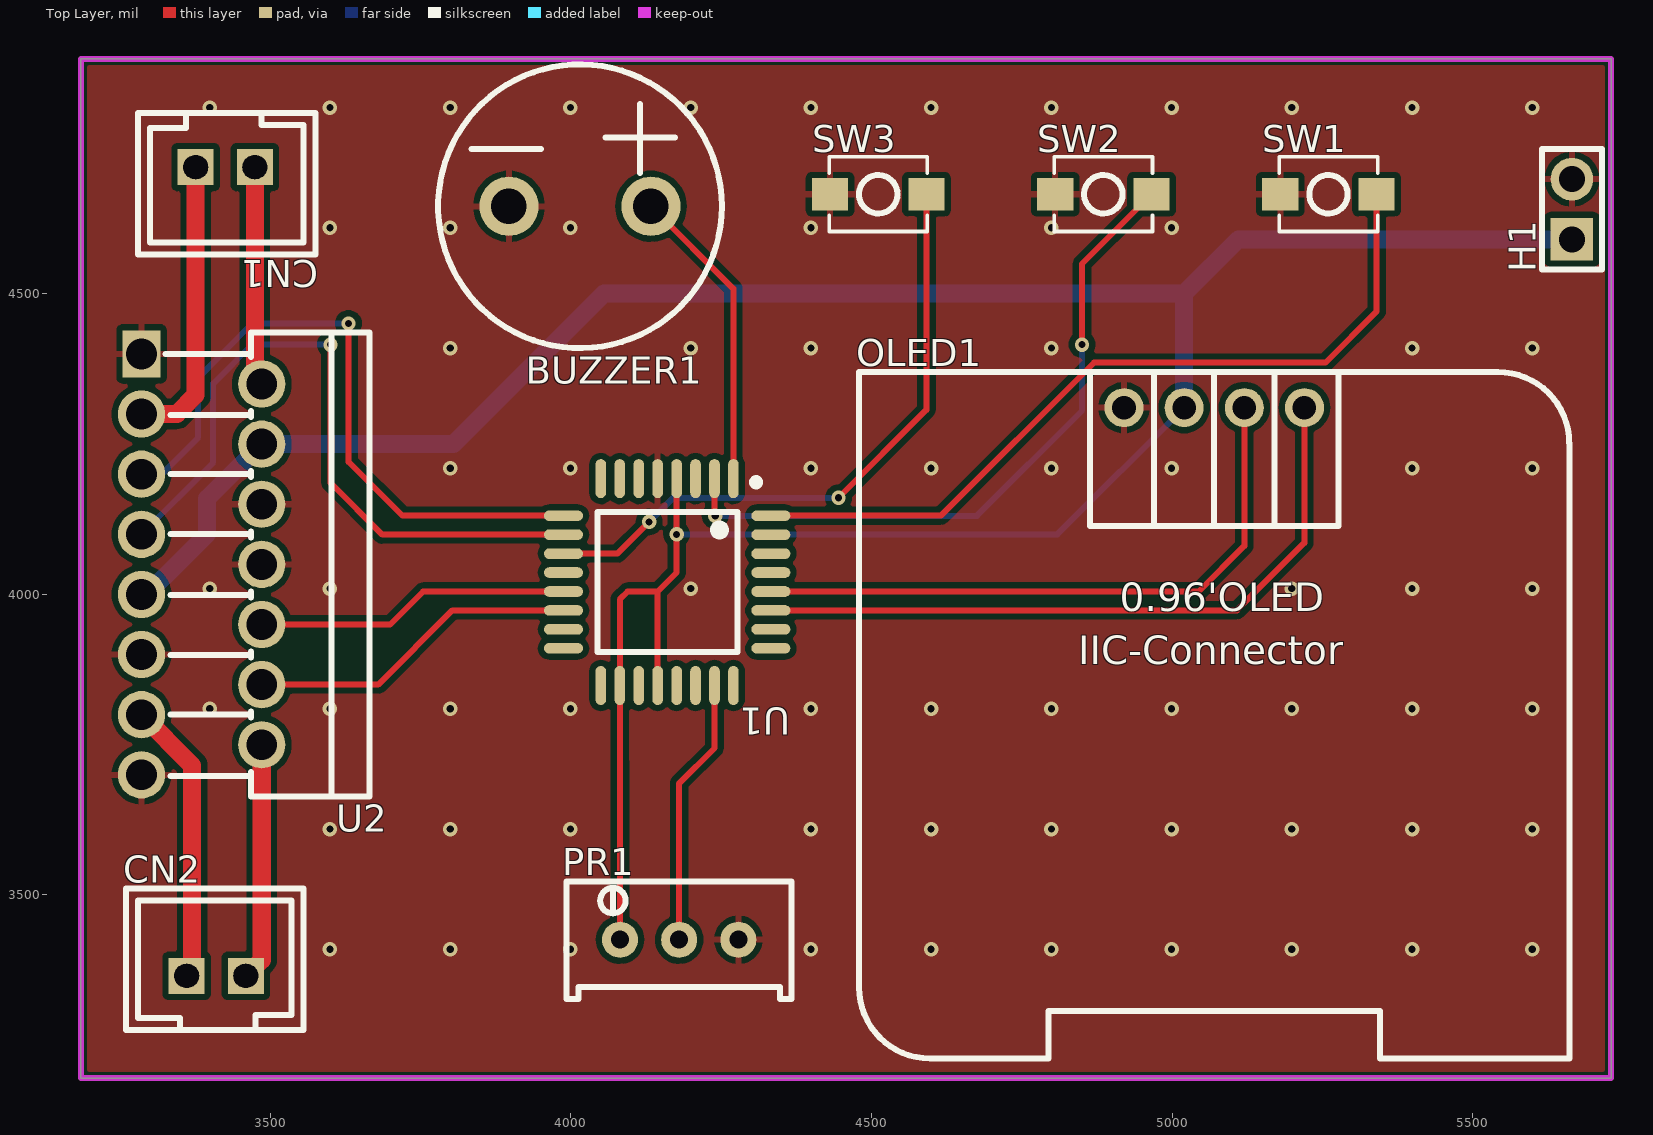
[diagram p0: Top Layer view]
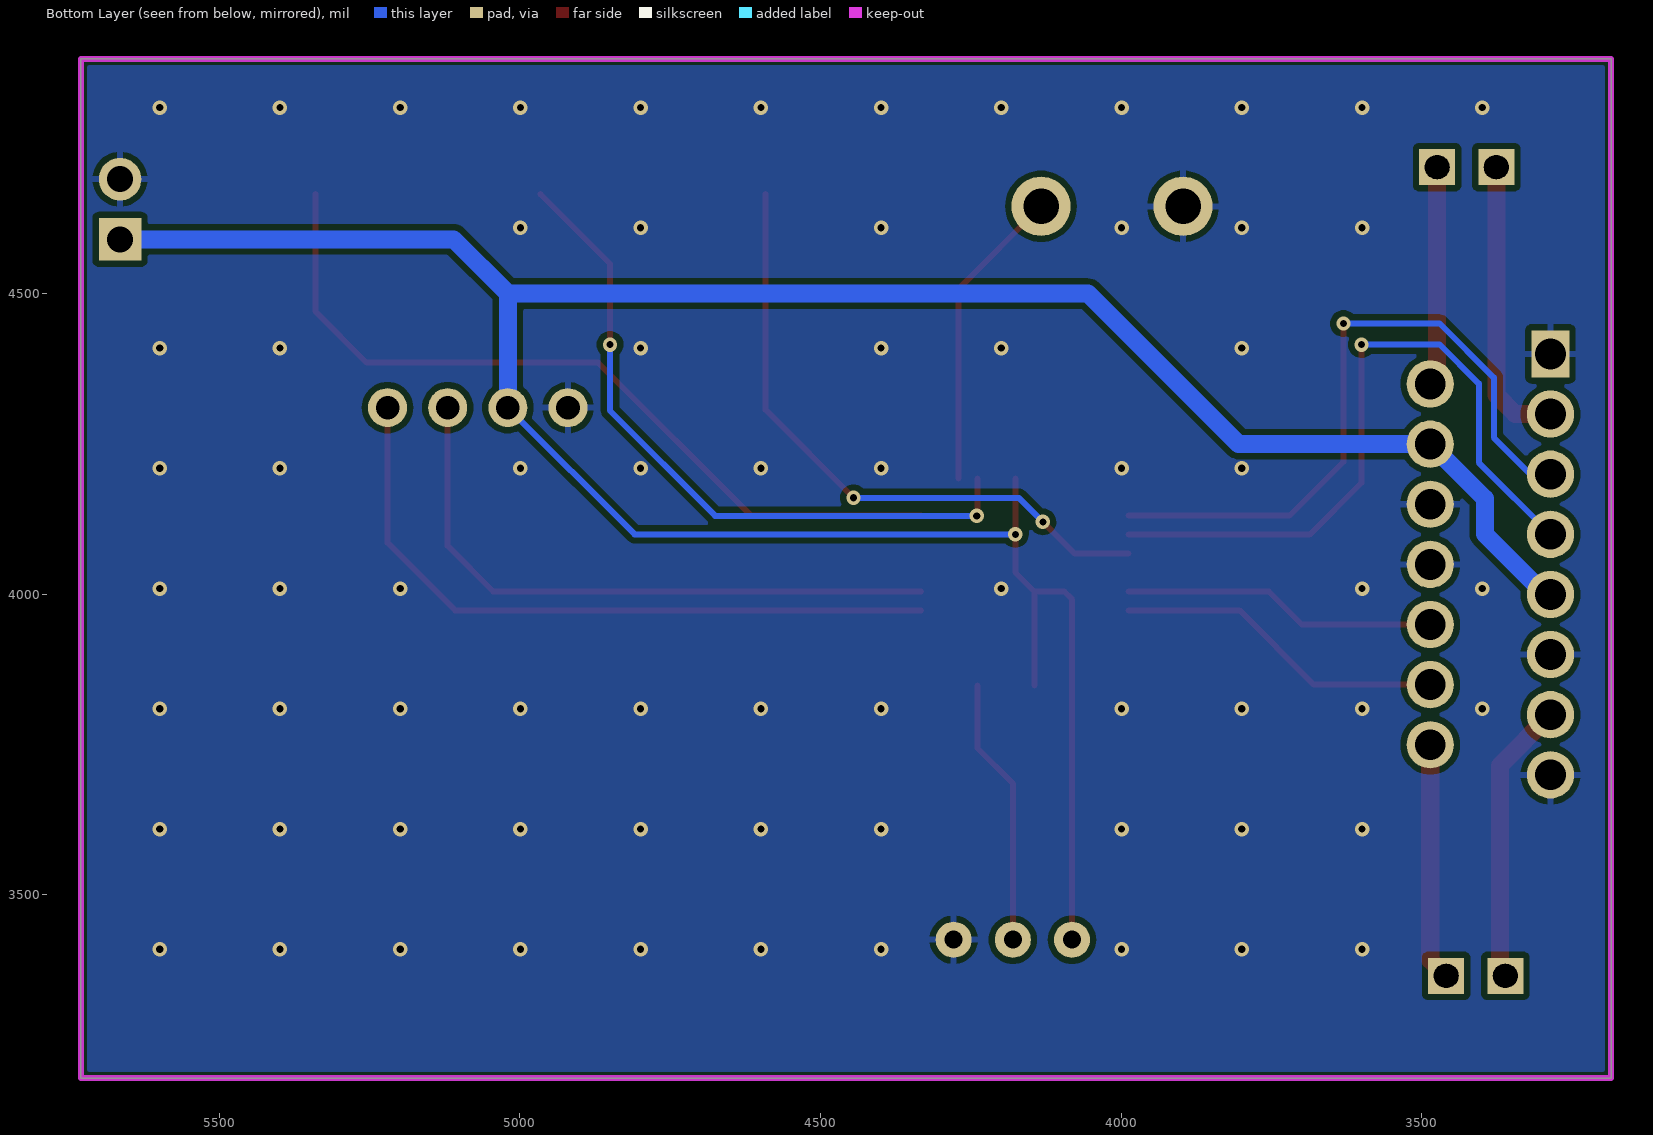
[diagram p1: Bottom Layer view, seen from below]
# Altium PCB MISC52152.pcbdoc
Units mil, origin at the board's own origin, x right, y up, seen from the top; angles counter-clockwise.
Board outline 2545 x 1695 mil, 2 copper layers (Top Layer, Bottom Layer), stack 62.206 mil thick; 11 components, 17 nets, 68 pads, 76 vias.

## Layer stack, top to bottom
Top Solder Mask Layer: solder mask 0.394, Dk 3.3
Top Layer: signal copper 1.379
Dielectric1: surface 59.449, FR4, Dk 4.5
Bottom Layer: signal copper 1.378
Bottom Solder Mask Layer: solder mask 0.394, Dk 3.3

## Board outline
3185,4890 3185,3195 5730,3195 5730,4890

## Design rules (kind name [scope] priority, off if disabled: settings)
BoardOutlineClearance copperThickness2oz_1 [All] p2 off: genericclearance=7.99 ignorepadtopadclearanceinfootprint=FALSE except(0: Arc-SplitContinuation Track-SplitContinuation SMDPad-SplitContinuation THPad-SplitContinuation Via-SplitContinuation Fill-SplitContinuation Region-SplitContinuation Poly-SplitContinuation Text-SplitContinuation Hole-SplitContinuation; 5.98: Arc-CutoutEdge SMDPad-CutoutEdge THPad-CutoutEdge Via-CutoutEdge Fill-CutoutEdge Region-CutoutEdge Text-CutoutEdge; 6.93: Hole-OutlineEdge Hole-CutoutEdge; 10: Poly-OutlineEdge Poly-CutoutEdge; 11.81: Arc-OutlineEdge Track-OutlineEdge SMDPad-OutlineEdge THPad-OutlineEdge Via-OutlineEdge Fill-OutlineEdge Region-OutlineEdge Text-OutlineEdge Track-CutoutEdge)
BoardOutlineClearance copperThickness1oz_1 [All] p4: genericclearance=4.02 ignorepadtopadclearanceinfootprint=FALSE except(0: Arc-SplitContinuation Track-SplitContinuation SMDPad-SplitContinuation THPad-SplitContinuation Via-SplitContinuation Fill-SplitContinuation Region-SplitContinuation Poly-SplitContinuation Text-SplitContinuation Hole-SplitContinuation; 6: SMDPad-CutoutEdge THPad-CutoutEdge Via-CutoutEdge Fill-CutoutEdge Region-CutoutEdge Text-CutoutEdge; 6.93: Hole-OutlineEdge Hole-CutoutEdge; 10: Poly-OutlineEdge Poly-CutoutEdge; 11.8: Arc-OutlineEdge Track-OutlineEdge SMDPad-OutlineEdge THPad-OutlineEdge Via-OutlineEdge Fill-OutlineEdge Region-OutlineEdge Text-OutlineEdge; 11.81: Arc-CutoutEdge Track-CutoutEdge)
Clearance copperThickness2oz [All] p1 off: gap=7.99 ignorepadtopadclearanceinfootprint=FALSE except(5.98: SMDPad-Track SMDPad-SMDPad THPad-Track SMDPad-THPad THPad-THPad Track-Via SMDPad-Via THPad-Via Via-Via Fill-Track Region-Track Fill-SMDPad Region-SMDPad Fill-THPad Region-THPad Fill-Via Region-Via Fill-Fill Fill-Region Region-Region Arc-Track Arc-SMDPad Arc-THPad Arc-Via Fill-Arc Region-Arc Arc-Arc Text-Track SMDPad-Text Text-THPad Text-Via Fill-Text Region-Text Arc-Text Text-Text; 6.93: Hole-Track Hole-SMDPad Hole-THPad Hole-Via Fill-Hole Region-Hole Hole-Arc Hole-Text; 10: Poly-Track Poly-SMDPad Poly-THPad Poly-Via Poly-Fill Poly-Region Poly-Poly Poly-Arc Poly-Text Poly-Hole)
Clearance copperThickness1oz [All] p3: gap=4.02 ignorepadtopadclearanceinfootprint=FALSE except(5.98: SMDPad-Track SMDPad-SMDPad THPad-Track SMDPad-THPad THPad-THPad Track-Via SMDPad-Via THPad-Via Via-Via Fill-Track Region-Track Fill-SMDPad Region-SMDPad Fill-THPad Region-THPad Fill-Via Region-Via Fill-Fill Fill-Region Region-Region; 6: Arc-Track Arc-SMDPad Arc-THPad Arc-Via Fill-Arc Region-Arc Arc-Arc Text-Track SMDPad-Text Text-THPad Text-Via Fill-Text Region-Text Arc-Text Text-Text; 6.93: Hole-Track Hole-SMDPad Hole-THPad Hole-Via Fill-Hole Region-Hole Hole-Arc Hole-Text; 10: Poly-Track Poly-SMDPad Poly-THPad Poly-Via Poly-Fill Poly-Region Poly-Poly Poly-Arc Poly-Text Poly-Hole)
DiffPairsRouting differentialPair [All] p1: maxlimit=6 minlimit=6 mostfreqgap=6 toplayer_minwidth=5 toplayer_prefwidth=10 toplayer_maxwidth=100 toplayer_mingap=6 toplayer_prefgap=6 toplayer_maxgap=6 bottomlayer_minwidth=5 bottomlayer_prefwidth=10 bottomlayer_maxwidth=100 bottomlayer_mingap=6 bottomlayer_prefgap=6 bottomlayer_maxgap=6 maxuncoupledlength=10
HoleToHoleClearance otherClearance [All] p1: gap=11.81 allowstackedmicrovias=TRUE
Length netLength [All] p1: minlimit=0 maxlimit=0
MatchedLengths netLengthTolerance [All] p1: tolerance=1000
PasteMaskExpansion pasteMaskExpansion [All] p1: expansion=0
PlaneConnect innerPlane [All] p1: planeconnectstyle=Relief reliefexpansion=20 reliefentries=4 reliefconductorwidth=10 reliefairgap=10
PolygonConnect copperRegion [(InNet('GND'))] p1: connectstyle=Relief reliefconductorwidth=10 reliefentries=4 polygonreliefangle="90 Angle" airgapwidth=10 via.connectstyle=Relief via.reliefconductorwidth=10 via.reliefentries=4 via.polygonreliefangle="90 Angle" via.airgapwidth=10
RoutingVias viaSize [All] p1: holewidth=12.01 width=24.02 viastyle="Through Hole" minholewidth=11.81 minwidth=19.68 maxholewidth=248.03 maxwidth=393.7
SolderMaskExpansion solderMaskExpansion [IsVia] p1: expansion=-1000 istentingtop=TRUE
SolderMaskExpansion solderMaskExpansion [All] p2: expansion=2 istentingtop=FALSE
Width copperThickness2oz_2 [All] p1 off: maxlimit=100 minlimit=8 preferedwidth=10
Width copperThickness1oz_2 [All] p2: maxlimit=100 minlimit=5 preferedwidth=10

## Components (designator, comment, footprint, x,y, rotation, side; value= is the part's Value field where it differs from the comment)
BUZZER1 "buzzer" BUZ-TH_BD12.0-P6.00-D0.9-RD 4015,4645 r0 top
CN1 "XH2.54-2PIN-直针" CONN-TH_XH2.54-2P 3424.99,4709.99 r180 top
CN2 "XH2.54-2PIN-直针" CONN-TH_XH2.54-2P 3410,3365 r0 top
H1 "" HDR-TH_2P-P2.54-V-M-1 5665,4640 r90 top
OLED1 "" 0.96OLED_4P 5070,4310 r0 top
PR1 "10kΩ" R_3296 4180,3430 r0 top
SW1 "" Key_SMD_3x4x2 5260,4665 r0 top
SW2 "" Key_SMD_3x4x2 4885.6,4665 r0 top
SW3 "" Key_SMD_3x4x2 4511.19,4665 r0 top
U1 "ATMEGA328PB-AUR" TQFP-32_L7.0-W7.0-P0.80-LS9.0-BL 4160,4020 r180 top
U2 "L298N" MULTIWATT-15_L19.6-W5.0-P1.27-L 3385.7,4049.36 r270 top

## Footprints (in the part's own frame and the unit in brackets; to place one, negate y for a bottom-side part, rotate by r counter-clockwise, add the part's x,y. Pads: shape width x height; smd on the part's side, far side on the other; paste and mask are expansions set on the pad)
0.96OLED_4P [mm]
  round 1.65 hole 1 copper offset 0,0: 1(-3.81,-0.001) 2(-1.27,0.002) 3(1.27,0.002) 4(3.81,0.002)
  silkscreen extent -15,-27.5 15,1.5
BUZ-TH_BD12.0-P6.00-D0.9-RD [mm]
  round 2.5 hole 1.5 paste+0 mask+0.05: 1(-3,0) 2(3,0)
  silkscreen extent -5.99,-5.99 5.99,5.99
CONN-TH_XH2.54-2P [mil]
  rect 60x60 hole 39.37 slot 41.34 at 0 deg paste+0 mask+1.97: 1(-49.22,0) 2(49.21,0)
  silkscreen extent -150,-90 145,145
HDR-TH_2P-P2.54-V-M-1 [mm]
  rect 1.8x1.8 hole 1.1: 1(-1.27,0)
  round 1.8 hole 1.1: 2(1.27,0)
  silkscreen extent -2.54,-1.27 2.54,1.27
Key_SMD_3x4x2 [mm]
  rect 1.53x1.36 smd paste+0 mask+0.051: 1(-2.035,0) 2(2.035,0)
  silkscreen extent -2.08,-1.58 2.08,1.58
MULTIWATT-15_L19.6-W5.0-P1.27-L [mm]
  rect 2x1.6 hole 1.3: 1(-8.89,-2.54)
  round 2 hole 1.3: 2(-7.62,2.54) 3(-6.35,-2.54) 4(-5.08,2.54) 5(-3.81,-2.54) 6(-2.54,2.54) 7(-1.27,-2.54) 8(0,2.54) 9(1.27,-2.54) 10(2.54,2.54) 11(3.81,-2.54) 12(5.08,2.54) 13(6.35,-2.54) 14(7.62,2.54) 15(8.89,-2.54)
  silkscreen extent -9.8,-1.52 9.8,7.09
R_3296 [mil]
  round 60 hole 30 paste+0 mask+2: 1(-98.4,-5) 2(0,-5) 3(98.4,-5)
  silkscreen extent -187,-103 187,92
TQFP-32_L7.0-W7.0-P0.80-LS9.0-BL [mm]
  oval 0.45x1.65 smd: 1(-2.8,-4.369) 2(-2,-4.369) 3(-1.2,-4.369) 4(-0.4,-4.369) 5(0.4,-4.369) 6(1.2,-4.369) 7(2,-4.369) 8(2.8,-4.369) 17(2.8,4.369) 18(2,4.369) 19(1.2,4.369) 20(0.4,4.369) 21(-0.4,4.369) 22(-1.2,4.369) 23(-2,4.369) 24(-2.8,4.369)
  oval 1.65x0.45 smd: 9(4.381,-2.8) 10(4.381,-2) 11(4.381,-1.2) 12(4.381,-0.4) 13(4.381,0.4) 14(4.381,1.2) 15(4.381,2) 16(4.381,2.8) 25(-4.381,2.8) 26(-4.381,2) 27(-4.381,1.2) 28(-4.381,0.4) 29(-4.381,-0.4) 30(-4.381,-1.2) 31(-4.381,-2) 32(-4.381,-2.8)
  silkscreen extent -3.91,-4.36 2.94,2.95

## Via types
v1: diameter 24.02, hole 12, Top Layer to Bottom Layer, 76 vias

## Nets (pads, with @x,y where several pads share a name; then routed paths per layer and width w, separated by ;. In a path a pad name is that pad's centre, name@x,y a point inside that pad or via, vN(x,y) a via of type N, cw(c..) or ccw(c..) an arc to the next point about the centre after c; other vN are vias at no path point)
$1N37: CN1.1 U2.2 | length 365.4
  Top Layer w30: CN1.1 3474.21,4360.85 U2.2
$1N38: CN1.2 U2.3 | length 482.3
  Top Layer w30: U2.3 3344.36,4299.36 3375.78,4330.78 CN1.2
$1N39: CN2.1 U2.13 | length 473.1
  Top Layer w30: U2.13 3370,3715.06 3370,3374.22 CN2.1
$1N40: CN2.2 U2.14 | length 395.3
  Top Layer w30: CN2.2 3485.7,3391.48 U2.14
+5V: H1.1 OLED1.2 PR1.1 U1.4 U1.18 U1.20 U2.4 U2.9 | length 4771.7
  Top Layer w10: PR1.1 4081.6,3720.92 4081.26,3721.26 U1.18 4081.26,3991.26 4094.25,4004.25 4144.25,4004.25 ; U1.20 4144.25,4004.25 ; U1.4 v1(4175.75,4099.25) 4175.75,4035.75 4144.25,4004.25
  Bottom Layer w10: v1(4175.75,4099.25) 4809.2,4099.25 OLED1.2@5020,4310.05
  Bottom Layer w30: U2.9 3294.36,3999.36 3395,4100 3395,4158.67 U2.4 3804.36,4249.36 4055,4500 5020,4500 ; OLED1.2@5020,4310.05 5020,4500 ; H1.1 5110,4590 5020,4500
BTN_MODE: SW2.2 U1.2 | length 1152.9
  Top Layer w10: U1.2 4238.74,4131.26 v1(4240,4130) ; v1(4850,4415) 4850,4549.28 SW2.2
  Bottom Layer w10: v1(4240,4130) 4675,4130 4850,4305 v1(4850,4415)
BTN_START: SW1.2 U1.32 | length 1343.3
  Top Layer w10: U1.32 4615.24,4130.24 4870,4385 5255,4385 5340.12,4470.12 SW1.2
BTN_STOP: SW3.2 U1.11 | length 1061.5
  Top Layer w10: U1.11 4077.24,4067.24 v1(4130,4120) ; v1(4445,4160) 4591.31,4306.31 SW3.2
  Bottom Layer w10: v1(4130,4120) 4170,4160 v1(4445,4160)
BUZZER: BUZZER1.2 U1.1 | length 509.8
  Top Layer w10: BUZZER1.2 4270.24,4507.87 U1.1
GND: BUZZER1.1 H1.2 OLED1.1 PR1.3 SW1.1 SW2.1 SW3.1 U1.5 U2.1 U2.6 U2.8 U2.11 U2.15
  other v1: 3599.1,3409.1 3799.1,3409.1 3999.1,3409.1 4399.1,3409.1 4599.1,3409.1 4799.1,3409.1 4999.1,3409.1 5199.1,3409.1 5399.1,3409.1 5599.1,3409.1 3599.1,3609.1 3799.1,3609.1 3999.1,3609.1 4399.1,3609.1 4599.1,3609.1 4799.1,3609.1 4999.1,3609.1 5199.1,3609.1 5399.1,3609.1 5599.1,3609.1 3399.1,3809.1 3599.1,3809.1 3799.1,3809.1 3999.1,3809.1 4399.1,3809.1 4599.1,3809.1 4799.1,3809.1 4999.1,3809.1 5199.1,3809.1 5399.1,3809.1 5599.1,3809.1 3399.1,4009.1 3599.1,4009.1 4199.1,4009.1 5199.1,4009.1 5399.1,4009.1 5599.1,4009.1 3799.1,4209.1 3999.1,4209.1 4399.1,4209.1 4599.1,4209.1 4799.1,4209.1 4999.1,4209.1 5399.1,4209.1 5599.1,4209.1 3799.1,4409.1 4199.1,4409.1 4399.1,4409.1 4799.1,4409.1 5399.1,4409.1 5599.1,4409.1 3599.1,4609.1 3799.1,4609.1 3999.1,4609.1 4399.1,4609.1 4799.1,4609.1 4999.1,4609.1 3399.1,4809.1 3599.1,4809.1 3799.1,4809.1 3999.1,4809.1 4199.1,4809.1 4399.1,4809.1 4599.1,4809.1 4799.1,4809.1 4999.1,4809.1 5199.1,4809.1 5399.1,4809.1 5599.1,4809.1
IN1: U1.9 U2.5 | length 1131.4
  Top Layer w10: v1(3630,4450) 3630,4220 3719.76,4130.24 U1.9
  Bottom Layer w10: U2.5 3319.36,4199.36 3380,4260 3380,4360 3470,4450 v1(3630,4450)
IN2: U1.10 U2.7 | length 1175.2
  Top Layer w10: v1(3600,4415) 3600,4185 3686.26,4098.74 U1.10
  Bottom Layer w10: U2.7 3405,4218.67 3405,4350 3470,4415 v1(3600,4415)
IN3: U1.13 U2.10 | length 524.5
  Top Layer w10: U2.10 3699.36,3949.36 3754.25,4004.25 U1.13
IN4: U1.14 U2.12 | length 552.9
  Top Layer w10: U2.12 3679.36,3849.36 3802.76,3972.76 U1.14
SCL: OLED1.3 U1.28 | length 1048.9
  Top Layer w10: U1.28 5044.25,4004.25 5120,4080 OLED1.3@5120,4310.05
SDA: OLED1.4 U1.27 | length 1159
  Top Layer w10: U1.27 5107.76,3972.76 5220,4085 OLED1.4@5220,4310.05
WATER: PR1.2 U1.23 | length 447.3
  Top Layer w10: PR1.2 4180,3685 4238.74,3743.74 U1.23
pads on no net: U1.3 U1.6 U1.7 U1.8 U1.12 U1.15 U1.16 U1.17 U1.19 U1.21 U1.22 U1.24 U1.25 U1.26 U1.29 U1.30 U1.31

## Polygon pours and split planes (outlines as drawn)
GND on Bottom Layer (solid, remove dead copper, pour order 2): 3000,5080 3000,3000 5870,3000 5870,5080
GND on Top Layer (solid, remove dead copper, pour order 0): 3070,5010 3070,3010 5850,3010 5850,5010

## Keep-outs
Board Outline Layer:
  the board outline again, w10